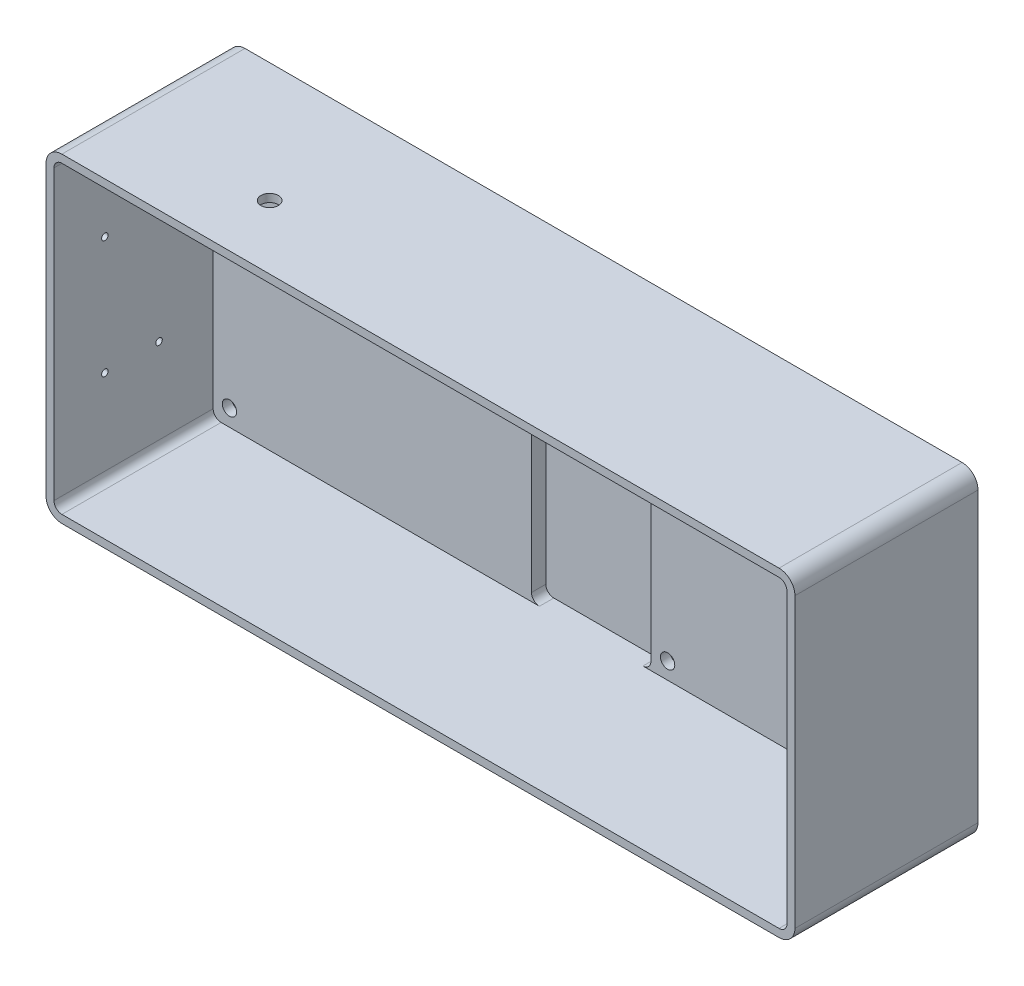
from build123d import *

# Parameters (mm, degrees)
BOSS_EXTRUDE1_DEPTH                                  = 115
SHELL1_T                                             = -5
SKETCH5_R                                            = 5.5
CUT_EXTRUDE4_DEPTH                                   = 10
SKETCH6_R                                            = 2.05
CUT_EXTRUDE5_DEPTH                                   = 10
FILLET1_R                                            = 10
FILLET2_R                                            = 5
BOSS_EXTRUDE2_DEPTH                                  = 10
HOLE_SIZE_PER_SOCKET_HEAD_CAP_SCREW_TYPE_D           = 9
HOLE_SIZE_PER_SOCKET_HEAD_CAP_SCREW_TYPE_CBORE_D     = 15
HOLE_SIZE_PER_SOCKET_HEAD_CAP_SCREW_TYPE_CBORE_DEPTH = 9
SKETCH10_W                                           = 75
SKETCH10_H                                           = 191
CUT_EXTRUDE6_DEPTH                                   = 9
FILLET3_R                                            = 5


with BuildPart() as part:
    # Sketch1 → Boss-Extrude1 (new body)
    with BuildSketch(Plane.XY):
        Polygon((285.5, 0), (285.5, -100.5), (185, -100.5), (-185, -100.5), (-185, 100.5), (185, 100.5), (285.5, 100.5), align=None)
    extrude(amount=BOSS_EXTRUDE1_DEPTH)

    # Shell1
    shell1_openings = [part.faces().sort_by_distance(p)[0] for p in [
        (50.25, 0, 115),
    ]]
    offset(amount=SHELL1_T, openings=shell1_openings, kind=Kind.INTERSECTION)

    # Sketch5 → Cut-Extrude4 (cut)
    with BuildSketch(Plane(origin=(-84.5, 100.5, 0), x_dir=(0, 0, 1), z_dir=(0, 1, 0))):
        with Locations((75, 0)):
            Circle(SKETCH5_R)
    extrude(amount=-CUT_EXTRUDE4_DEPTH, mode=Mode.SUBTRACT)

    # Sketch6 → Cut-Extrude5 (cut)
    with BuildSketch(Plane.ZY.offset(185)):
        with Locations(Location((49, -37, 0), (0, 0, 270))):
            Circle(SKETCH6_R)
        with Locations(Location((49, 37, 0), (0, 0, 270))):
            Circle(SKETCH6_R)
        with Locations(Location((83, 37, 0), (0, 0, 270))):
            Circle(SKETCH6_R)
        with Locations(Location((83, -37, 0), (0, 0, 270))):
            Circle(SKETCH6_R)
    extrude(amount=-CUT_EXTRUDE5_DEPTH, mode=Mode.SUBTRACT)

    # Fillet1
    fillet1_edges = [part.edges().sort_by_distance(p)[0] for p in [
        (-185, -100.5, 57.5),
        (-185, 100.5, 57.5),
        (285.5, 100.5, 57.5),
        (285.5, -100.5, 57.5),
    ]]
    fillet(fillet1_edges, radius=FILLET1_R)

    # Fillet2
    fillet2_edges = [part.edges().sort_by_distance(p)[0] for p in [
        (280.5, -95.5, 60),
        (280.5, 95.5, 60),
        (-180, 95.5, 60),
        (-180, -95.5, 60),
    ]]
    fillet(fillet2_edges, radius=FILLET2_R)

    # Sketch7 → Boss-Extrude2 (add)
    with BuildSketch(Plane.XY.offset(5)):
        with BuildLine():
            Line((280.5, -90.5), (280.5, 90.5))
            ThreePointArc((280.5, 90.5), (279.035533906, 94.035533906), (275.5, 95.5))
            Line((275.5, 95.5), (-175, 95.5))
            ThreePointArc((-175, 95.5), (-178.535533906, 94.035533906), (-180, 90.5))
            Line((-180, 90.5), (-180, -90.5))
            ThreePointArc((-180, -90.5), (-178.535533906, -94.035533906), (-175, -95.5))
            Line((-175, -95.5), (275.5, -95.5))
            ThreePointArc((275.5, -95.5), (279.035533906, -94.035533906), (280.5, -90.5))
        make_face()
    extrude(amount=BOSS_EXTRUDE2_DEPTH)

    # Hole size per socket head cap screw type1 (through all)
    with Locations(Plane(origin=(0, 0, 0), x_dir=(-1, 0, 0), z_dir=(0, 0, -1))):
        with Locations((-270.25, -85), (-270.25, 85), (169.75, 85), (169.75, -85), (-105.5, -85), (-105.5, 85)):
            CounterBoreHole(HOLE_SIZE_PER_SOCKET_HEAD_CAP_SCREW_TYPE_D / 2, HOLE_SIZE_PER_SOCKET_HEAD_CAP_SCREW_TYPE_CBORE_D / 2, HOLE_SIZE_PER_SOCKET_HEAD_CAP_SCREW_TYPE_CBORE_DEPTH)

    # Sketch10 → Cut-Extrude6 (cut)
    with BuildSketch(Plane.XY.offset(15)):
        with Locations((57.5, 0)):
            Rectangle(SKETCH10_W, SKETCH10_H)
    extrude(amount=-CUT_EXTRUDE6_DEPTH, mode=Mode.SUBTRACT)

    # Fillet3
    fillet3_edges = [part.edges().sort_by_distance(p)[0] for p in [
        (20, -95.5, 10.5),
        (20, 95.5, 10.5),
        (95, 95.5, 10.5),
        (95, -95.5, 10.5),
    ]]
    fillet(fillet3_edges, radius=FILLET3_R)


solid = part.part
